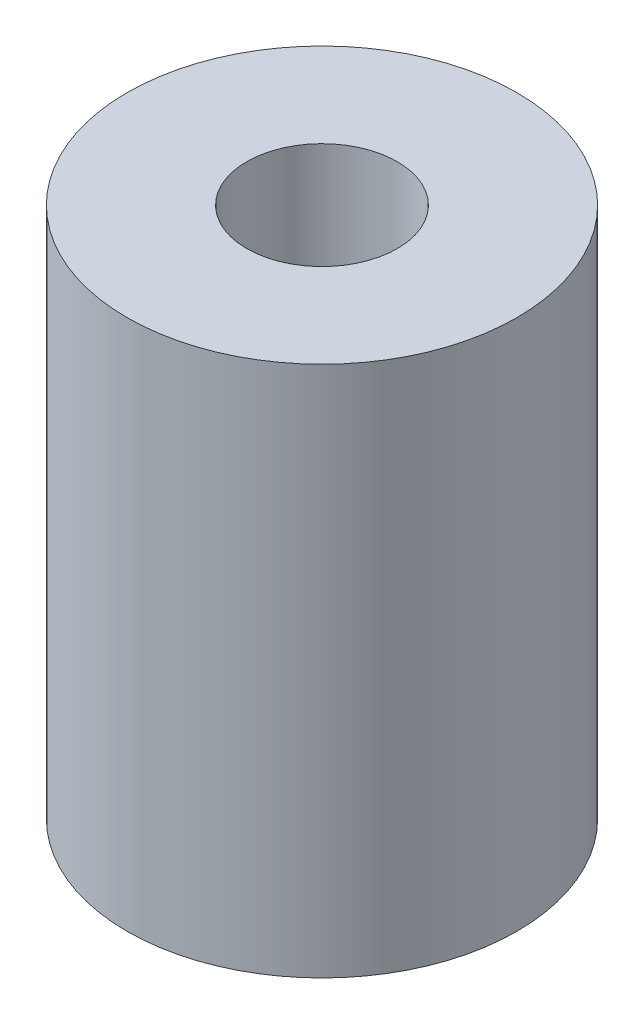
SolidWorks part; units mm, degrees
material "SS400B"
ref_plane "Front Plane" through (0, 0, 0) normal (0, 0, 1) x (1, 0, 0)
ref_plane "Top Plane" through (0, 0, 0) normal (0, 1, 0) x (1, 0, 0)
ref_plane "Right Plane" through (0, 0, 0) normal (1, 0, 0) x (0, 0, -1)
sketch "Sketch1" plane through (0, 0, 0) normal (0, 1, 0) x (1, 0, 0)
  circle A0 centre (0, 0) radius 11
  dimension "D1" = 22
extrude "Boss-Extrude1" add sketch "Sketch1" along normal blind 30
hole_wizard "M10 Tapped Hole1" positions "Sketch2" profile "Sketch3" tap size "M10" standard "GB"
sketch "Sketch2" plane through (0, 30, 0) normal (0, 1, 0) x (1, 0, 0)
  point P0 (0, 0)
sketch "Sketch3" plane through (0, 30, 0) normal (1, 0, 0) x (0, 0, 1)
  line L0 (0, 0) -> (0, 37.5537)
  line L1 (0, 37.5537) -> (4.25, 35)
  line L2 (4.25, 35) -> (4.25, 0)
  line L5 (4.25, 0) -> (0, 0)
  line L10 (0, 37.5537) -> (-4.25, 35) construction
  line L11 (0, -6.35) -> (0, 107.95) construction
  dimension "螺纹孔钻头直径" = 8.5
  dimension "螺纹孔钻头深度" = 35
  dimension "导头角度" = 118
cosmetic thread "Cosmetic thread1"
